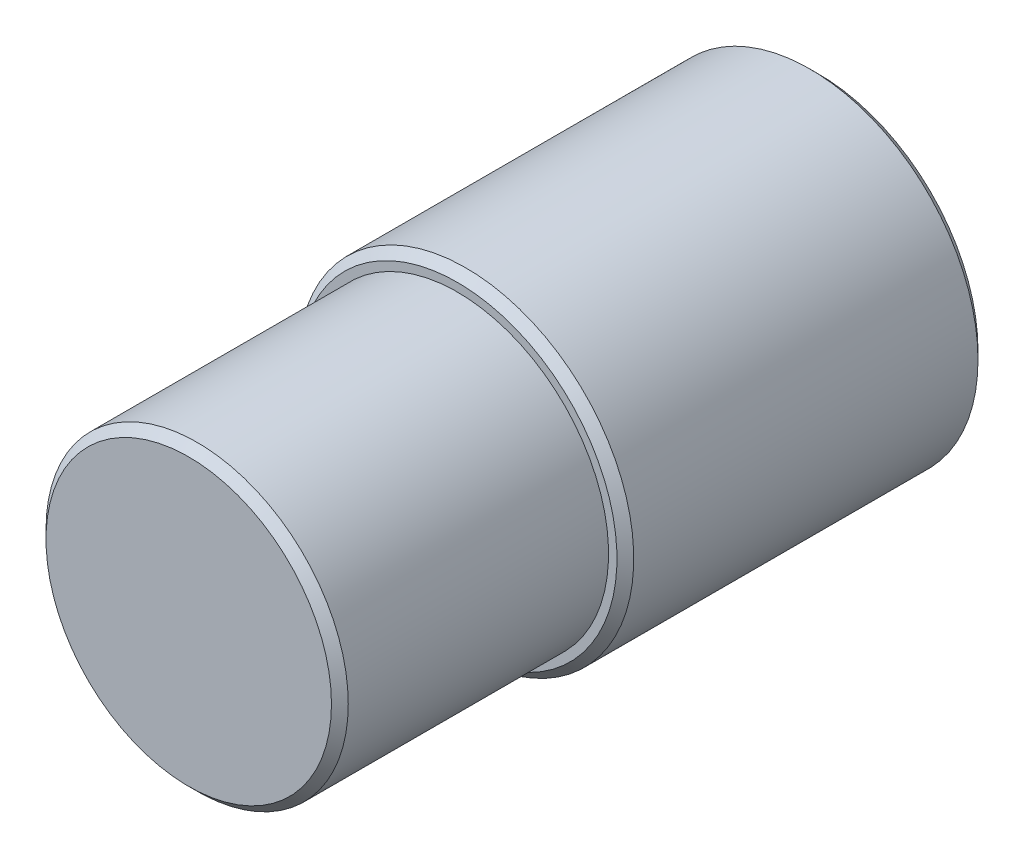
SolidWorks part; units mm, degrees
ref_plane "Front Plane" through (0, 0, 0) normal (0, 0, 1) x (1, 0, 0)
ref_plane "Top Plane" through (0, 0, 0) normal (0, 1, 0) x (1, 0, 0)
ref_plane "Right Plane" through (0, 0, 0) normal (1, 0, 0) x (0, 0, -1)
sketch "Sketch1" plane through (0, 0, 0) normal (0, 0, 1) x (1, 0, 0)
  circle A0 centre (0, 0) radius 9
  dimension "D1" = 18
extrude "Boss-Extrude1" add sketch "Sketch1" along normal blind 37.5
sketch "Sketch2" plane through (0, 0, 0) normal (0, 0, -1) x (-1, 0, 0)
  circle A0 centre (0, 0) radius 10
  dimension "D1" = 20
extrude "Boss-Extrude2" add sketch "Sketch2" against normal blind 21.5
chamfer "Chamfer1" distance 0.5 angle 45 3 edges at (9, 0, 37.5) (-10, 0, 0) (-10, 0, 21.5)
